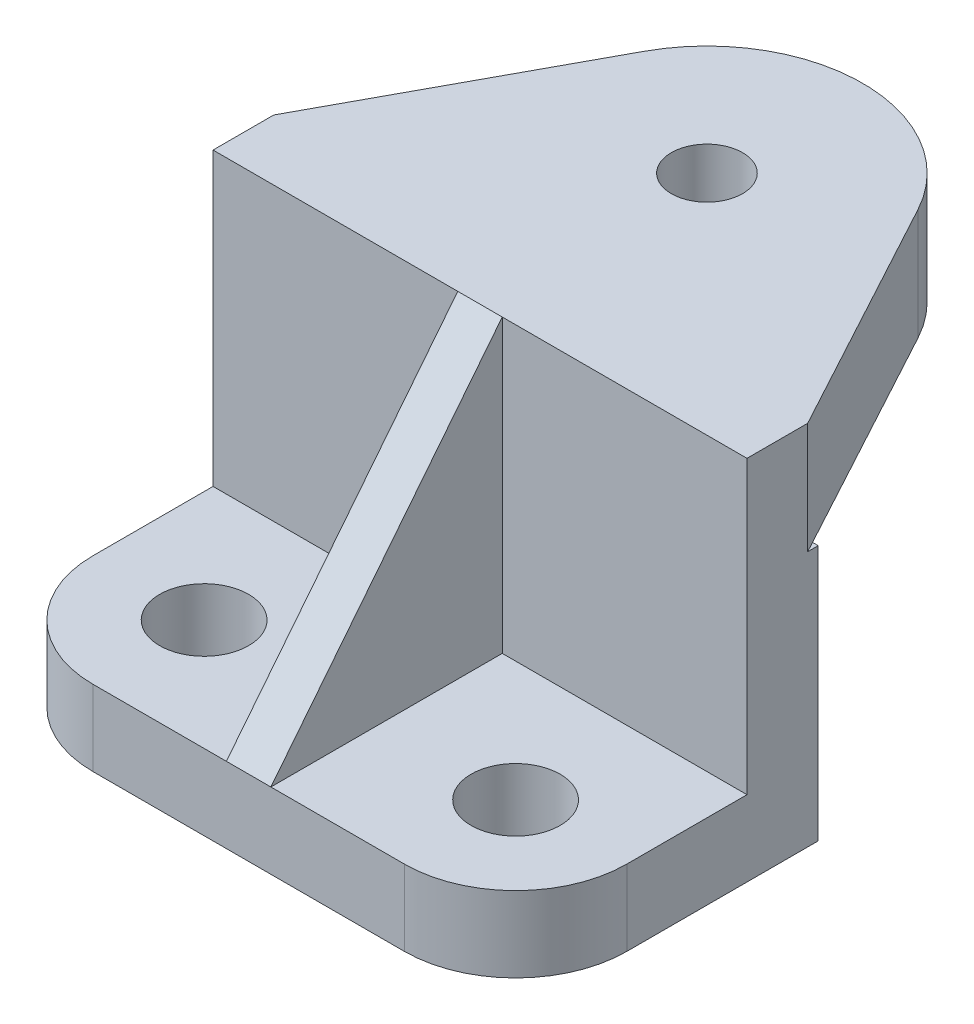
SolidWorks part; units mm, degrees
ref_plane "Front Plane" through (0, 0, 0) normal (0, 0, 1) x (1, 0, 0)
ref_plane "Top Plane" through (0, 0, 0) normal (0, 1, 0) x (1, 0, 0)
ref_plane "Right Plane" through (0, 0, 0) normal (1, 0, 0) x (0, 0, -1)
sketch "Sketch1" plane through (0, 0, 0) normal (1, 0, 0) x (0, 0, -1)
  line L0 (0, 0) -> (68, 0)
  line L1 (68, 0) -> (68, 82.4712)
  line L2 (68, 82.4712) -> (52, 82.4712)
  line L3 (52, 82.4712) -> (52, 17)
  line L4 (52, 17) -> (0, 17)
  line L5 (0, 17) -> (0, 0)
  line L6 (52, 82.4712) -> (0, 17)
  dimension "D1" = 17
  dimension "D2" = 16
  dimension "D3" = 68
extrude "Boss-Extrude1" add sketch "Sketch1" against normal blind 120 contours L3 L6 L4 | L4 L5 L0 L1 L2 L3
sketch "Sketch2" plane through (0, 0, 0) normal (1, 0, 0) x (0, 0, -1)
  line L0 (52, 82.4712) -> (0, 17)
  line L1 (0, 17) -> (52, 17)
  line L2 (52, 17) -> (52, 82.4712)
extrude "Cut-Extrude1" cut sketch "Sketch2" against normal blind 55
sketch "Sketch3" plane through (-120, 0, 0) normal (-1, 0, 0) x (0, 0, 1)
  line L0 (-52, 82.4712) -> (0, 17)
  line L1 (0, 17) -> (-52, 17)
  line L2 (-52, 17) -> (-52, 82.4712)
extrude "Cut-Extrude2" cut sketch "Sketch3" against normal blind 55
sketch "Sketch5" plane through (0, 0, 0) normal (0, -1, 0) x (1, 0, 0)
  line L0 (-120, 0) -> (-120, -25)
  line L1 (-120, 0) -> (-120, -68) construction
  line L2 (-120, -25) -> (-95, -25)
  line L3 (-95, -25) -> (-25, -25)
  circle A0 centre (-95, -25) radius 10
  circle A1 centre (-25, -25) radius 10
  circle A2 centre (-95, -25) radius 25
  circle A3 centre (-25, -25) radius 25
extrude "Cut-Extrude3" cut sketch "Sketch5" against normal blind 55
sketch "Sketch6" plane through (0, 0, 0) normal (1, 0, 0) x (0, 0, -1)
  line L0 (68, 82.4712) -> (138, 82.4712)
  line L1 (138, 82.4712) -> (138, 57.4712)
  line L2 (138, 57.4712) -> (68, 57.4712)
  line L3 (68, 0) -> (68, 82.4712) construction
  line L4 (68, 57.4712) -> (68, 82.4712)
extrude "Boss-Extrude2" add sketch "Sketch6" against normal blind 120
sketch "Sketch7" plane through (0, 82.4712, 0) normal (0, 1, 0) x (1, 0, 0)
  line L2 (-120, 138) -> (0, 138) construction
  line L5 (-120, 52) -> (-120, 65.6493)
  line L6 (-120, 138) -> (-120, 52) construction
  line L7 (-60, 138) -> (-60, 138.8474)
  line L8 (0, 138) -> (0, 52) construction
  line L9 (-120, 65.6493) -> (-90.7839, 119.6539)
  line L10 (0, 65.6493) -> (-29.2161, 119.6539)
  circle A0 centre (-60, 103) radius 8
  arc A1 (-29.2161, 119.6539) -> (-90.7839, 119.6539) centre (-60, 103) ccw
  line M1 (0, 52) -> (0, 138)
  line M2 (0, 138) -> (-120, 138)
  line M3 (-120, 138) -> (-120, 52)
extrude "Cut-Extrude4" cut sketch "Sketch7" against normal blind 25 contours A0 | A1 L10 M1 M2 | A1 L9 M2 M3
